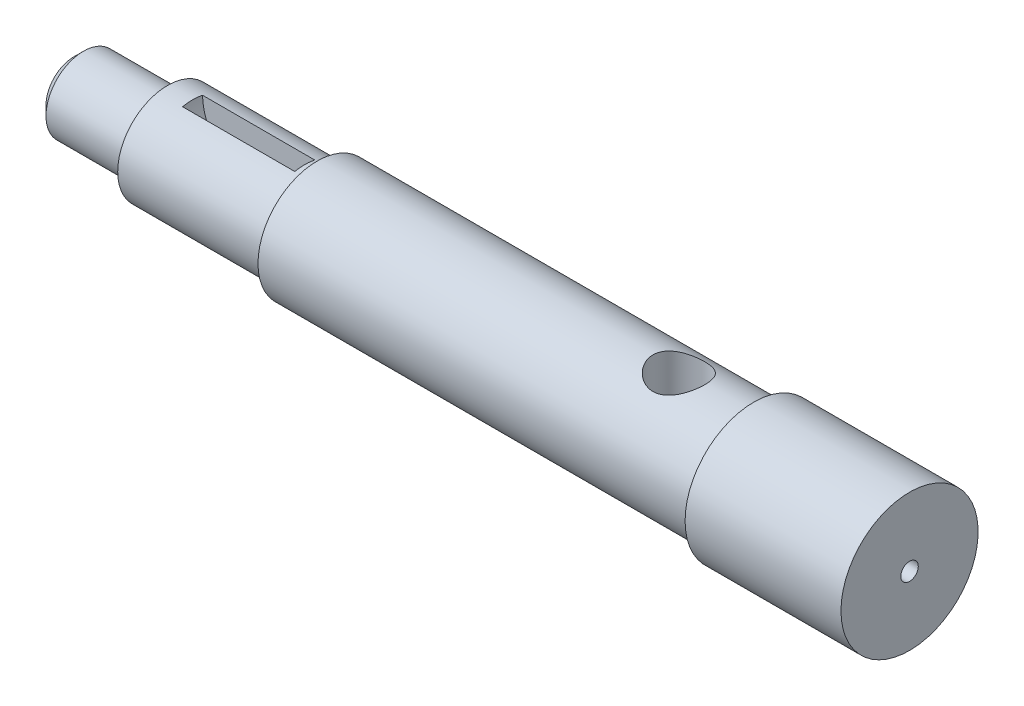
SolidWorks part; units mm, degrees
ref_plane "Front Plane" through (0, 0, 0) normal (0, 0, 1) x (1, 0, 0)
ref_plane "Top Plane" through (0, 0, 0) normal (0, 1, 0) x (1, 0, 0)
ref_plane "Right Plane" through (0, 0, 0) normal (1, 0, 0) x (0, 0, -1)
sketch "Sketch1" plane through (0, 0, 0) normal (0, 1, 0) x (1, 0, 0)
  line L0 (-52.3736, 0) -> (81.6264, 0) construction
  line L1 (-52.3736, 0) -> (-52.3736, 6)
  line L2 (-52.3736, 6) -> (-37.3736, 6)
  line L3 (-37.3736, 6) -> (-37.3736, 8)
  line L4 (-37.3736, 8) -> (-13.3736, 8)
  line L5 (-13.3736, 8) -> (-13.3736, 9.5)
  line L6 (-13.3736, 9.5) -> (56.6264, 9.5)
  line L7 (56.6264, 9.5) -> (56.6264, 11)
  line L8 (56.6264, 11) -> (81.6264, 11)
  line L9 (81.6264, 11) -> (81.6264, 0)
  line L10 (-52.3736, 0) -> (81.6264, 0)
  dimension "D1" = 134
  dimension "D2" = 25
  dimension "D3" = 70
  dimension "D4" = 24
  dimension "D5" = 6
  dimension "D6" = 2
  dimension "D7" = 1.5
  dimension "D8" = 11
revolve "Revolve1" add sketch "Sketch1" angle 360 about L0
sketch "Sketch2" plane through (81.6264, 0, 0) normal (1, 0, 0) x (0, 0, -1)
  circle A0 centre (0, 0) radius 1.4
extrude "Cut-Extrude1" cut sketch "Sketch2" against normal blind 44
sketch "Sketch3" plane through (0, 0, 0) normal (0, 1, 0) x (1, 0, 0)
  circle A0 centre (44.6264, 0) radius 4.15
  dimension "D1" = 8.3
extrude "Cut-Extrude2" cut sketch "Sketch3" against normal through all and the other way through all
ref_plane "Plane1" through (0, 8, 0) normal (0, 1, 0) x (-1, 0, 0)
sketch "Sketch5" plane through (0, 8, 0) normal (0, 1, 0) x (-1, 0, 0)
  line L0 (24.3736, 1.6) -> (24.3736, -1.6) construction
  line L2 (24.3736, 1.6) -> (24.3736, -1.6)
  line L3 (15.3736, 1.6) -> (24.3736, 1.6)
  line L4 (15.3736, 1.6) -> (15.3736, -1.6)
  line L5 (15.3736, -1.6) -> (24.3736, -1.6)
revolve "Cut-Revolve3" cut sketch "Sketch5" angle 360 about L0
chamfer "Chamfer1" distance 1.5 angle 45 1 edges at (-52.3736, 0, 6)
